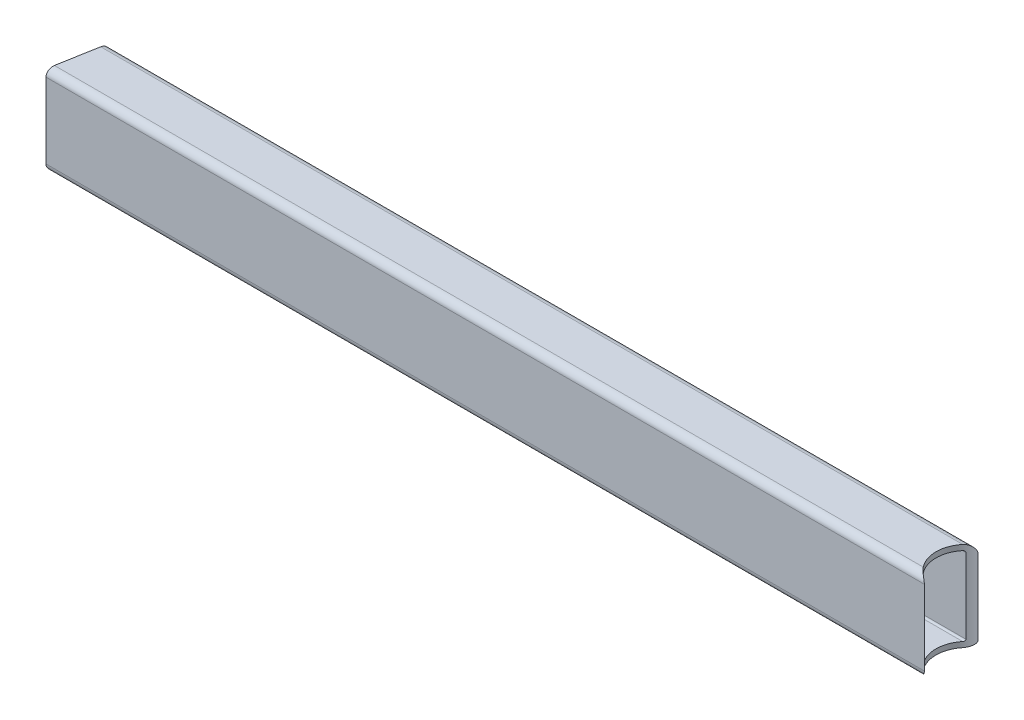
SolidWorks part; units mm, degrees
material "1023 碳钢板 (SS)"
ref_plane "Front Plane" through (0, 0, 0) normal (0, 0, 1) x (1, 0, 0)
ref_plane "Top Plane" through (0, 0, 0) normal (0, 1, 0) x (1, 0, 0)
ref_plane "Right Plane" through (0, 0, 0) normal (1, 0, 0) x (0, 0, -1)
sketch "草图1" plane through (0, 0, 0) normal (0, 0, 1) x (1, 0, 0)
  line L0 (0, 0) -> (-600, 0)
  dimension "D3" = 600
other "Square tube 30 X 30 X 2.6(15)"
ref_plane "Plane2" through (0, 0, 0) normal (-1, 0, 0) x (0, -1, 0)
sketch "Sketch1" plane through (0, 0, 0) normal (-1, 0, 0) x (0, -1, 0)
  line L0 (-21, -12) -> (21, -12)
  line L1 (-22, -11) -> (-22, 11)
  line L2 (21, 12) -> (-21, 12)
  line L3 (22, 11) -> (22, -11)
  line L4 (-21, -15) -> (21, -15)
  line L5 (-25, -11) -> (-25, 11)
  line L6 (21, 15) -> (-21, 15)
  line L7 (25, 11) -> (25, -11)
  arc A0 (25, 11) -> (21, 15) centre (21, 11) ccw
  arc A1 (21, -15) -> (25, -11) centre (21, -11) ccw
  arc A2 (-25, -11) -> (-21, -15) centre (-21, -11) ccw
  arc A3 (-21, 15) -> (-25, 11) centre (-21, 11) ccw
  arc A4 (-21, 12) -> (-22, 11) centre (-21, 11) ccw
  arc A5 (22, 11) -> (21, 12) centre (21, 11) ccw
  arc A6 (21, -12) -> (22, -11) centre (21, -11) ccw
  arc A7 (-22, -11) -> (-21, -12) centre (-21, -11) ccw
  point P0 (-25, 0)
  point P1 (25, 0)
  point P2 (0, 15)
  point P3 (0, -15)
  point P4 (0, 0)
  point P5 (-25, -15)
  point P6 (25, -15)
  point P7 (25, 15)
  point P8 (-25, 15)
  point P33 (0, 0)
  dimension "D1" = 4
  dimension "D2" = 50
  dimension "Thickness" = 3
  dimension "V_leg" = 30
sketch "Sketch12" plane through (0, -25, 0) normal (0, -1, 0) x (1, 0, 0)
  line L0 (-500, 15) -> (-494.7102, -15)
  line L4 (-600, 15) -> (0, 15) construction
  line L5 (-600, -15) -> (0, -15) construction
  line L6 (-494.7102, -15) -> (-600, -15)
  line L7 (-600, -15) -> (-600, 15)
  line L8 (-600, 15) -> (-500, 15)
  dimension "D1" = 80
  dimension "D2" = 500
extrude "Cut-Extrude3" cut sketch "Sketch12" against normal blind 113
sketch "Sketch13" plane through (0, -25, 0) normal (0, -1, 0) x (1, 0, 0)
  circle A0 centre (0, 0) radius 17.5
  dimension "D1" = 35
extrude "Cut-Extrude4" cut sketch "Sketch13" against normal blind 113
